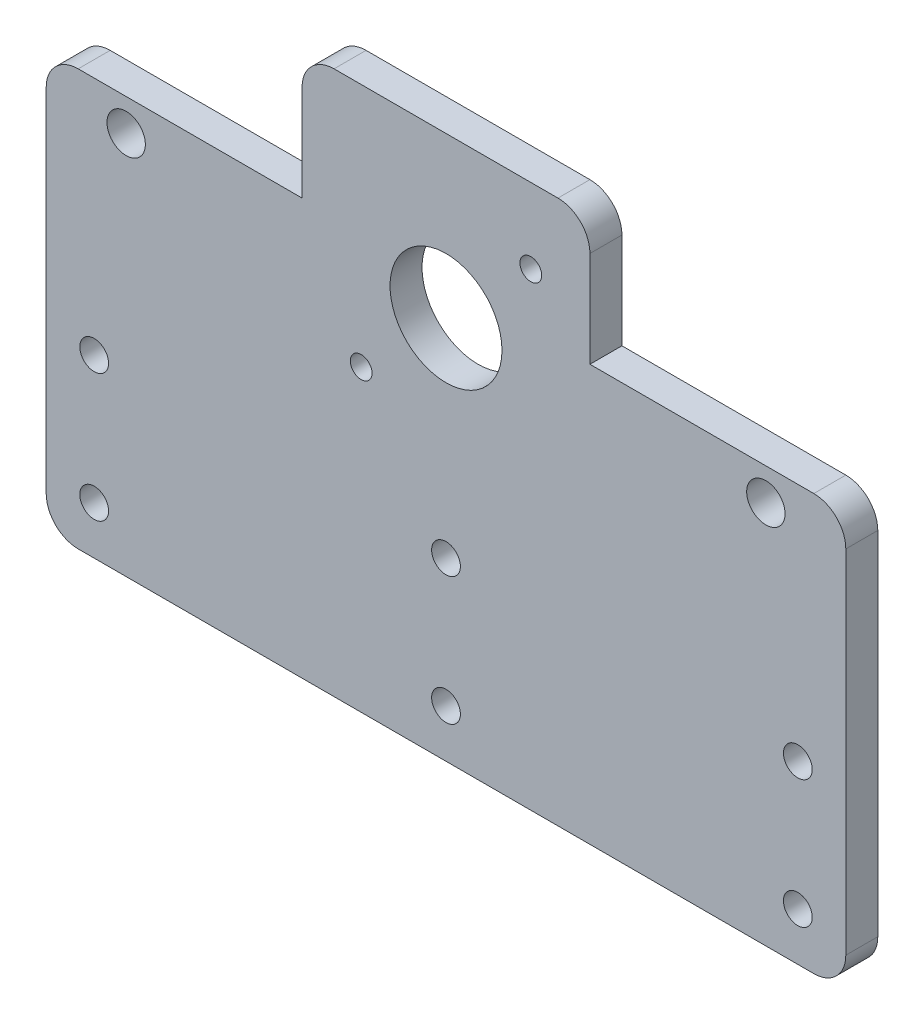
SolidWorks part; units mm, degrees
ref_plane "前视基准面" through (0, 0, 0) normal (0, 0, 1) x (1, 0, 0)
ref_plane "上视基准面" through (0, 0, 0) normal (0, 1, 0) x (1, 0, 0)
ref_plane "右视基准面" through (0, 0, 0) normal (1, 0, 0) x (0, 0, -1)
sketch "草图1" plane through (0, 0, 0) normal (0, 0, 1) x (1, 0, 0)
  line L1 (-125, 85) -> (125, 85)
  line L2 (-125, 85) -> (-125, -85)
  line L3 (-125, -85) -> (125, -85)
  line L4 (125, 85) -> (125, -85)
  line L5 (-125, 85) -> (125, -85) construction
  line L6 (-125, -85) -> (125, 85) construction
  point P0 (0, 0)
  dimension "D1" = 250
  dimension "D2" = 170
extrude "凸台-拉伸1" add sketch "草图1" along normal mid plane 10
sketch "草图2" plane through (0, 0, 5) normal (0, 0, 1) x (1, 0, 0)
  line L0 (125, 85) -> (-125, 85) construction
  line L1 (45, 85) -> (125, 85)
  line L2 (45, 85) -> (45, 45)
  line L3 (45, 45) -> (125, 45)
  line L4 (125, 85) -> (125, 45)
  line L5 (125, -85) -> (125, 85) construction
  dimension "D1" = 80
  dimension "D2" = 40
extrude "切除-拉伸1" cut sketch "草图2" against normal blind 10
mirror "镜向1" about plane through (0, 0, 0) normal (1, 0, 0) of "切除-拉伸1"
hole_wizard "Ø9.0 (9) 直径孔1" positions "草图4" profile "草图3" hole size "Ø9.0" standard "GB" end condition up to next
sketch "草图4" plane through (0, 0, 5) normal (0, 0, 1) x (1, 0, 0)
  line L0 (-125, -85) -> (125, -85) construction
  line L1 (-125, 45) -> (-125, -85) construction
  point P0 (-110, -30)
  point P2 (-110, -70)
  dimension "D1" = 15
  dimension "D2" = 40
  dimension "D3" = 15
sketch "草图3" plane through (-110, -30, 5) normal (1, 0, 0) x (0, -1, 0)
  line L0 (0, 0) -> (0, 10)
  line L1 (0, 10) -> (4.5, 10)
  line L2 (4.5, 10) -> (4.5, 0)
  line L5 (4.5, 0) -> (0, 0)
  line L11 (0, -6.35) -> (0, 107.95) construction
  dimension "通孔孔直径" = 9
  dimension "通孔孔深度" = 10
pattern_linear "阵列(线性)1" count 3 spacing 110 along (1, 0, 0) of "Ø9.0 (9) 直径孔1"
hole_wizard "Ø12.0 (12) 直径孔1" positions "草图6" profile "草图5" hole size "Ø12.0" standard "GB" end condition up to next
sketch "草图6" plane through (0, 0, 5) normal (0, 0, 1) x (1, 0, 0)
  line L0 (-125, -85) -> (125, -85) construction
  point P0 (-100, 35)
  point P2 (100, 35)
  dimension "D1" = 200
  dimension "D2" = 100
  dimension "D3" = 120
sketch "草图5" plane through (-100, 35, 5) normal (1, 0, 0) x (0, -1, 0)
  line L0 (0, 0) -> (0, 10)
  line L1 (0, 10) -> (6, 10)
  line L2 (6, 10) -> (6, 0)
  line L5 (6, 0) -> (0, 0)
  line L11 (0, -6.35) -> (0, 107.95) construction
  dimension "通孔孔直径" = 12
  dimension "通孔孔深度" = 10
sketch "草图7" plane through (0, 0, 5) normal (0, 0, 1) x (1, 0, 0)
  line L0 (-125, -85) -> (125, -85) construction
  circle A0 centre (0, 35) radius 17.5
  dimension "D1" = 35
  dimension "D2" = 120
extrude "切除-拉伸2" cut sketch "草图7" against normal blind 10
hole_wizard "M8 螺纹孔1" positions "草图9" profile "草图8" tap size "M8" standard "ISO" end condition up to next
sketch "草图9" plane through (0, 0, 5) normal (0, 0, 1) x (1, 0, 0)
  circle A1 centre (0, 35) radius 17.5 construction
  point P0 (-26.515, 8.485)
  point P2 (26.515, 61.515)
  dimension "D1" = 53.03
  dimension "D2" = 53.03
  dimension "D3" = 26.515
  dimension "D4" = 26.515
sketch "草图8" plane through (-26.515, 8.485, 5) normal (1, 0, 0) x (0, -1, 0)
  line L0 (0, 0) -> (0, 10)
  line L1 (0, 10) -> (3.4, 10)
  line L2 (3.4, 10) -> (3.4, 0)
  line L5 (3.4, 0) -> (0, 0)
  line L11 (0, -6.35) -> (0, 107.95) construction
  dimension "通孔螺纹孔钻头直径" = 6.8
  dimension "通孔螺纹孔钻头深度" = 10
cosmetic thread "孔螺蚊线1" parameters "D2"=8
cosmetic thread "孔螺蚊线2" parameters "D2"=8
fillet "圆角1" radius 10 6 edges at (125, -85, 0) (125, 45, 0) (45, 85, 0) (-45, 85, 0) (-125, -85, 0) (-125, 45, 0)
